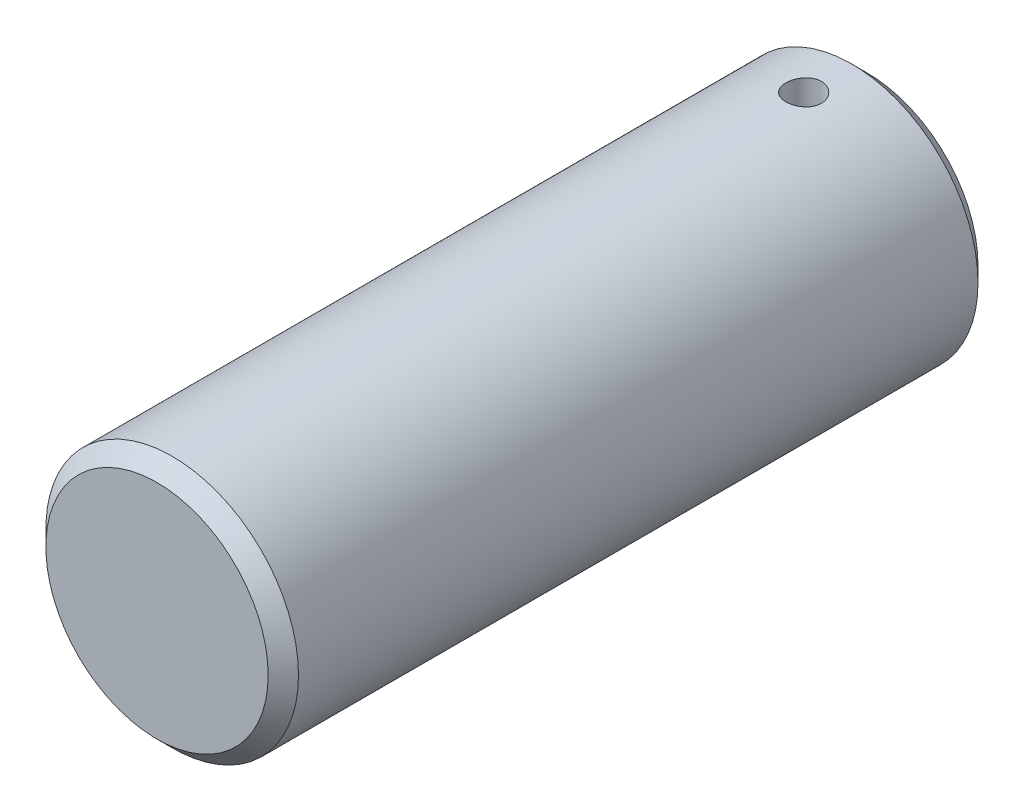
from build123d import *

# Parameters (mm, degrees)
SKETCH1_R               = 12.7
BOSS_EXTRUDE1_DEPTH     = 71.37
CHAMFER1_SIZE           = 1.524
CUT_EXTRUDE1_DEPTH      = 74.59522335
CUT_EXTRUDE1_DEPTH_BACK = 74.59522335
SKETCH2_R               = 1.785


with BuildPart() as part:
    # Sketch1 → Boss-Extrude1 (new body)
    with BuildSketch(Plane.XY):
        Circle(SKETCH1_R)
    extrude(amount=BOSS_EXTRUDE1_DEPTH)

    # Chamfer1
    chamfer1_edges = [part.edges().sort_by_distance(p)[0] for p in [
        (-12.7, 0, 0),
        (-12.7, 0, 71.37),
    ]]
    chamfer(chamfer1_edges, length=CHAMFER1_SIZE)

    # Sketch2 → Cut-Extrude1 (cut, two sides: drawn at the far end of the back side and taken through both)
    with BuildSketch(Plane(origin=(0, 0, 0), x_dir=(1, 0, 0), z_dir=(0, 1, 0)).offset(-CUT_EXTRUDE1_DEPTH_BACK)):
        with Locations(Location((0, -6.35, 0), (0, 0, 270))):
            Circle(SKETCH2_R)
    extrude(amount=CUT_EXTRUDE1_DEPTH + CUT_EXTRUDE1_DEPTH_BACK, mode=Mode.SUBTRACT)


solid = part.part
